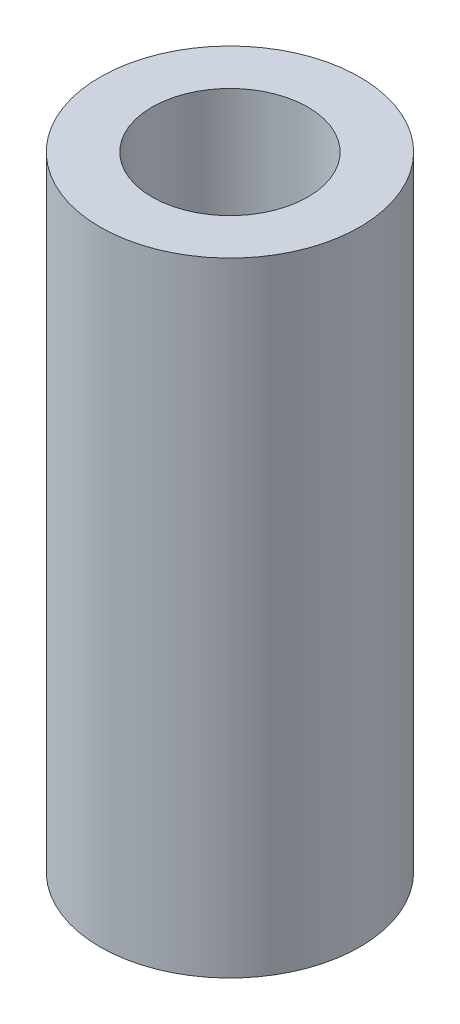
from build123d import *

# Parameters (mm, degrees)
SKETCH_1_R      = 2.5
SKETCH_1_R_2    = 1.5
EXTRUDE_1_DEPTH = 12


with BuildPart() as part:
    # 草图1 → 凸台-拉伸1 (new body)
    with BuildSketch(Plane(origin=(0, 0, 0), x_dir=(1, 0, 0), z_dir=(0, 1, 0))):
        with Locations(Location((0, 0, 0), (0, 0, 270))):
            Circle(SKETCH_1_R)
        with Locations(Location((0, 0, 0), (0, 0, 270))):
            Circle(SKETCH_1_R_2, mode=Mode.SUBTRACT)
    extrude(amount=EXTRUDE_1_DEPTH)


solid = part.part
